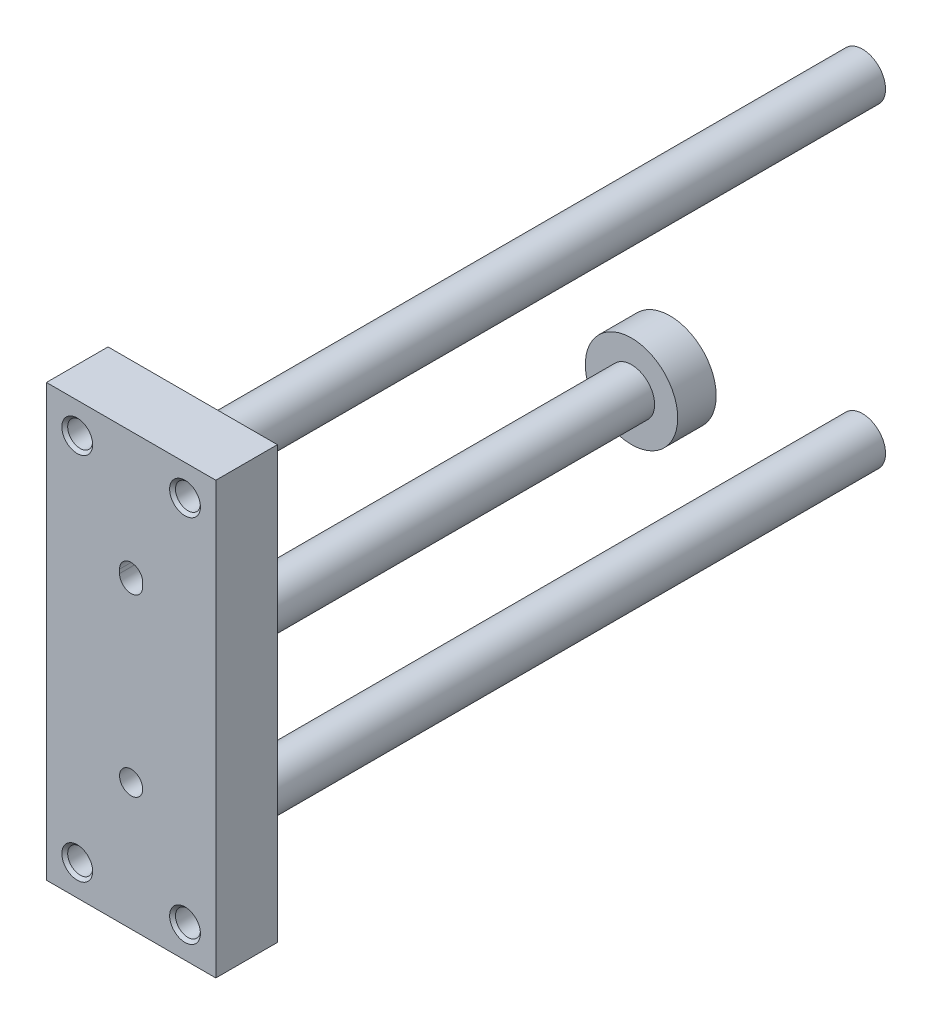
from build123d import *

# Parameters (mm, degrees)
SKETCH_1_W          = 22
SKETCH_1_H          = 56
EXTRUDE_1_DEPTH     = 8
CUT_EXTRUDE_1_DEPTH = 3
SKETCH_9_R          = 3
EXTRUDE_2_DEPTH     = 87
SKETCH_10_R         = 3
EXTRUDE_3_DEPTH     = 87
SKETCH_11_R         = 3
EXTRUDE_4_DEPTH     = 59.5
SKETCH_12_R         = 6
EXTRUDE_5_DEPTH     = 5


with BuildPart() as part:
    # 草图1 → 凸台-拉伸1 (new body)
    with BuildSketch(Plane.XY):
        Rectangle(SKETCH_1_W, SKETCH_1_H)
    extrude(amount=-EXTRUDE_1_DEPTH)

    # 草图2 → 切除-旋转1 (revolve, cut)
    with BuildSketch(Plane(origin=(0, 24, 0), x_dir=(1, 0, 0), z_dir=(0, 1, 0)), mode=Mode.PRIVATE) as cut_revolve_1_sk:
        Polygon((-7, 0), (-9, 0), (-8.621, 0.379), (-8.621, 7.621), (-9, 8), (-7, 8), align=None)
    revolve(cut_revolve_1_sk.sketch.rotate(Axis((-7, 24, -8), (0, 0, 1)), 180), axis=Axis((-7, 24, -8), (0, 0, 1)), mode=Mode.SUBTRACT)

    # 草图3 → 切除-旋转2 (revolve, cut)
    with BuildSketch(Plane(origin=(0, -24, 0), x_dir=(1, 0, 0), z_dir=(0, 1, 0)), mode=Mode.PRIVATE) as cut_revolve_2_sk:
        Polygon((-7, 0), (-9, 0), (-8.621, 0.379), (-8.621, 7.621), (-9, 8), (-7, 8), align=None)
    revolve(cut_revolve_2_sk.sketch.rotate(Axis((-7, -24, -8), (0, 0, 1)), 180), axis=Axis((-7, -24, -8), (0, 0, 1)), mode=Mode.SUBTRACT)

    # 草图4 → 切除-旋转3 (revolve, cut)
    with BuildSketch(Plane(origin=(0, -24, 0), x_dir=(1, 0, 0), z_dir=(0, 1, 0)), mode=Mode.PRIVATE) as cut_revolve_3_sk:
        Polygon((7, 0), (5, 0), (5.379, 0.379), (5.379, 7.621), (5, 8), (7, 8), align=None)
    revolve(cut_revolve_3_sk.sketch.rotate(Axis((7, -24, -8), (0, 0, 1)), 180), axis=Axis((7, -24, -8), (0, 0, 1)), mode=Mode.SUBTRACT)

    # 草图5 → 切除-旋转4 (revolve, cut)
    with BuildSketch(Plane(origin=(0, 24, 0), x_dir=(1, 0, 0), z_dir=(0, 1, 0)), mode=Mode.PRIVATE) as cut_revolve_4_sk:
        Polygon((7, 0), (5, 0), (5.379, 0.379), (5.379, 7.621), (5, 8), (7, 8), align=None)
    revolve(cut_revolve_4_sk.sketch.rotate(Axis((7, 24, -8), (0, 0, 1)), 180), axis=Axis((7, 24, -8), (0, 0, 1)), mode=Mode.SUBTRACT)

    # 草图6 → 切除-旋转5 (revolve, cut)
    with BuildSketch(Plane(origin=(0, 0, 0), x_dir=(0, 0, -1), z_dir=(1, 0, 0)), mode=Mode.PRIVATE) as cut_revolve_5_sk:
        Polygon((0, 11.5), (0, 13), (6, 13), (6.866025404, 11.5), align=None)
    revolve(cut_revolve_5_sk.sketch.rotate(Axis((0, 11.5, -6.866025404), (0, 0, 1)), 270), axis=Axis((0, 11.5, -6.866025404), (0, 0, 1)), mode=Mode.SUBTRACT)

    # 草图7 → 切除-旋转6 (revolve, cut)
    with BuildSketch(Plane(origin=(0, 0, 0), x_dir=(0, 0, -1), z_dir=(1, 0, 0)), mode=Mode.PRIVATE) as cut_revolve_6_sk:
        Polygon((0, -11.5), (0, -10), (6, -10), (6.866025404, -11.5), align=None)
    revolve(cut_revolve_6_sk.sketch.rotate(Axis((0, -11.5, -6.866025404), (0, 0, 1)), 270), axis=Axis((0, -11.5, -6.866025404), (0, 0, 1)), mode=Mode.SUBTRACT)

    # 草图8 → 切除-拉伸1 (cut)
    with BuildSketch(Plane.XY):
        with BuildLine():
            Line((1.5, 11.25), (1.5, 11.75))
            ThreePointArc((1.5, 11.75), (0, 13.25), (-1.5, 11.75))
            Line((-1.5, 11.75), (-1.5, 11.25))
            ThreePointArc((-1.5, 11.25), (0, 9.75), (1.5, 11.25))
        make_face()
    extrude(amount=-CUT_EXTRUDE_1_DEPTH, mode=Mode.SUBTRACT)

    # 草图9 → 凸台-拉伸2 (add)
    with BuildSketch(Plane.XY.offset(-8)):
        with Locations((0, 20.5)):
            Circle(SKETCH_9_R)
    extrude(amount=-EXTRUDE_2_DEPTH)

    # 草图10 → 凸台-拉伸3 (add)
    with BuildSketch(Plane.XY.offset(-8)):
        with Locations((0, -20.5)):
            Circle(SKETCH_10_R)
    extrude(amount=-EXTRUDE_3_DEPTH)

    # 草图11 → 凸台-拉伸4 (add)
    with BuildSketch(Plane.XY.offset(-8)):
        Circle(SKETCH_11_R)
    extrude(amount=-EXTRUDE_4_DEPTH)

    # 草图12 → 凸台-拉伸5 (add)
    with BuildSketch(Plane.XY.offset(-70)):
        Circle(SKETCH_12_R)
    extrude(amount=EXTRUDE_5_DEPTH)


solid = part.part
